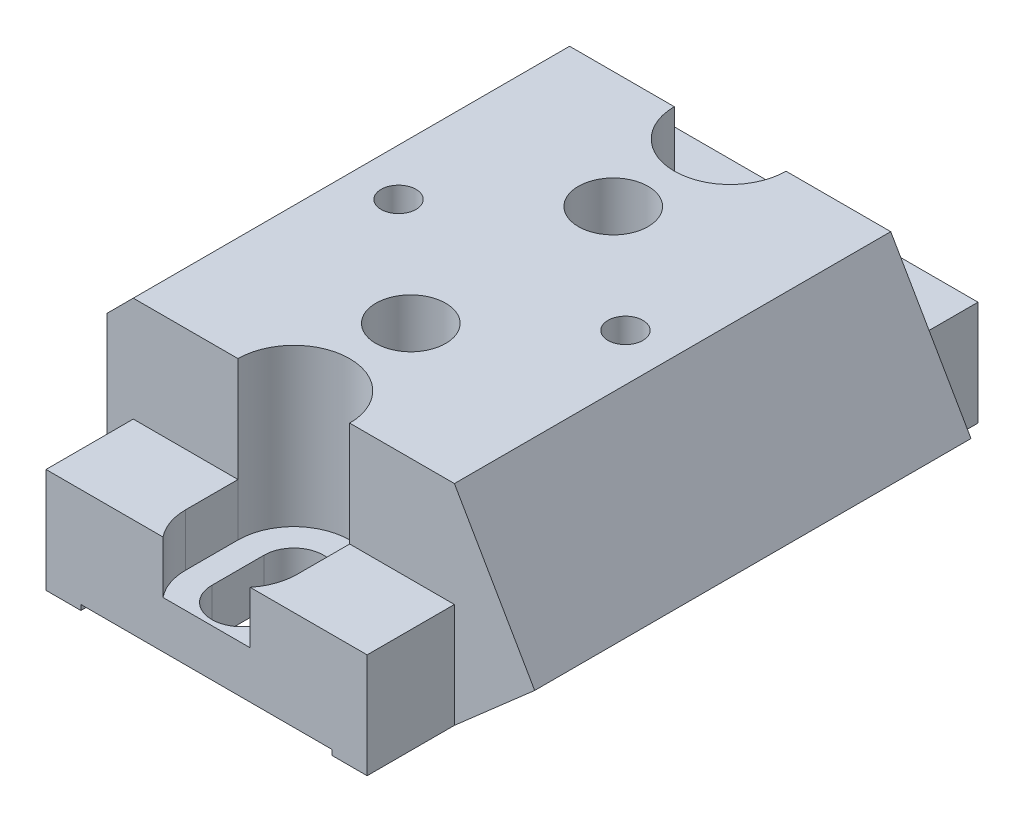
from build123d import *

# Parameters (mm, degrees)
SKETCH1_W           = 25
SKETCH1_H           = 12
BOSS_EXTRUDE1_DEPTH = 25
CUT_EXTRUDE1_DEPTH  = 30
CHAMFER1_SIZE       = 2
SKETCH5_W           = 21
SKETCH5_H           = 35
BOSS_EXTRUDE2_DEPTH = 6
SKETCH6_W           = 2.6
SKETCH6_H           = 5
CUT_EXTRUDE2_DEPTH  = 10
SKETCH11_W          = 14.4
SKETCH11_H          = 0.3
CUT_EXTRUDE5_DEPTH  = 48
CUT_EXTRUDE6_DEPTH  = 48
SKETCH15_W          = 25
SKETCH15_H          = 12
CUT_EXTRUDE8_DEPTH  = 0.5
SKETCH17_R          = 2
CUT_EXTRUDE10_DEPTH = 5
SKETCH18_R          = 1
CUT_EXTRUDE11_DEPTH = 4
CUT_EXTRUDE12_DEPTH = 17
CUT_EXTRUDE13_DEPTH = 9


with BuildPart() as part:
    # Sketch1 → Boss-Extrude1 (new body)
    with BuildSketch(Plane.XY):
        with Locations((12.5, -6)):
            Rectangle(SKETCH1_W, SKETCH1_H)
    extrude(amount=BOSS_EXTRUDE1_DEPTH)

    # Sketch2 → Cut-Extrude1 (cut)
    with BuildSketch(Plane.XY.offset(25)):
        Polygon((25, 0), (25, -7.967433715), (20.4, 0), align=None)
    extrude(amount=-CUT_EXTRUDE1_DEPTH, mode=Mode.SUBTRACT)

    # Chamfer1
    chamfer1_edges = [part.edges().sort_by_distance(p)[0] for p in [
        (0, 0, 12.5),
        (25, -12, 12.5),
        (0, -12, 12.5),
    ]]
    chamfer(chamfer1_edges, length=CHAMFER1_SIZE)

    # Sketch5 → Boss-Extrude2 (add)
    with BuildSketch(Plane.XZ.offset(12)):
        with Locations((12.5, 12.5)):
            Rectangle(SKETCH5_W, SKETCH5_H)
    extrude(amount=-BOSS_EXTRUDE2_DEPTH)

    # Sketch6 → Cut-Extrude2 (cut)
    with BuildSketch(Plane(origin=(0, -6, 0), x_dir=(1, 0, 0), z_dir=(0, 1, 0))):
        with Locations((21.7, -27.5)):
            Rectangle(SKETCH6_W, SKETCH6_H)
        with Locations((21.7, 2.5)):
            Rectangle(SKETCH6_W, SKETCH6_H)
    extrude(amount=-CUT_EXTRUDE2_DEPTH, mode=Mode.SUBTRACT)

    # Sketch11 → Cut-Extrude5 (cut)
    with BuildSketch(Plane.XY.offset(30)):
        with Locations((11.2, -11.85)):
            Rectangle(SKETCH11_W, SKETCH11_H)
    extrude(amount=-CUT_EXTRUDE5_DEPTH, mode=Mode.SUBTRACT)

    # Sketch12 → Cut-Extrude6 (cut)
    with BuildSketch(Plane.XY.offset(30)):
        Polygon((25, -7.967433715), (20.4, -12), (25.592855108, -12), align=None)
    extrude(amount=-CUT_EXTRUDE6_DEPTH, mode=Mode.SUBTRACT)

    # Sketch15 → Cut-Extrude8 (cut)
    with BuildSketch(Plane.ZY):
        with Locations((12.5, -6)):
            Rectangle(SKETCH15_W, SKETCH15_H)
    extrude(amount=-CUT_EXTRUDE8_DEPTH, mode=Mode.SUBTRACT)

    # Sketch17 → Cut-Extrude10 (cut)
    with BuildSketch(Plane(origin=(0, 0, 0), x_dir=(1, 0, 0), z_dir=(0, 1, 0))):
        with Locations(Location((11.2, -6.7, 0), (0, 0, 270))):
            Circle(SKETCH17_R)
        with Locations(Location((11.2, -18.3, 0), (0, 0, 270))):
            Circle(SKETCH17_R)
    extrude(amount=-CUT_EXTRUDE10_DEPTH, mode=Mode.SUBTRACT)

    # Sketch18 → Cut-Extrude11 (cut)
    with BuildSketch(Plane(origin=(0, 0, 0), x_dir=(1, 0, 0), z_dir=(0, 1, 0))):
        with Locations(Location((4.7, -12.5, 0), (0, 0, 270))):
            Circle(SKETCH18_R)
        with Locations(Location((17.7, -12.5, 0), (0, 0, 270))):
            Circle(SKETCH18_R)
    extrude(amount=-CUT_EXTRUDE11_DEPTH, mode=Mode.SUBTRACT)

    # Sketch19 → Cut-Extrude12 (cut)
    with BuildSketch(Plane(origin=(0, 0, 0), x_dir=(1, 0, 0), z_dir=(0, 1, 0))):
        with BuildLine():
            Line((12.9, -25), (12.9, -28))
            ThreePointArc((12.9, -28), (11.2, -29.7), (9.5, -28))
            Line((9.5, -28), (9.5, -25))
            ThreePointArc((9.5, -25), (11.2, -23.3), (12.9, -25))
        make_face()
        with BuildLine():
            Line((12.9, 0), (12.9, 3))
            ThreePointArc((12.9, 3), (11.2, 4.7), (9.5, 3))
            Line((9.5, 3), (9.5, 0))
            ThreePointArc((9.5, 0), (11.2, -1.7), (12.9, 0))
        make_face()
    extrude(amount=-CUT_EXTRUDE12_DEPTH, mode=Mode.SUBTRACT)

    # Sketch20 → Cut-Extrude13 (cut)
    with BuildSketch(Plane(origin=(0, 0, 0), x_dir=(1, 0, 0), z_dir=(0, 1, 0))):
        with BuildLine():
            Line((14.4, -25), (14.4, -28))
            ThreePointArc((14.4, -28), (11.2, -31.2), (8, -28))
            Line((8, -28), (8, -25))
            ThreePointArc((8, -25), (11.2, -21.8), (14.4, -25))
        make_face()
        with BuildLine():
            Line((14.4, 0), (14.4, 3))
            ThreePointArc((14.4, 3), (11.2, 6.2), (8, 3))
            Line((8, 3), (8, 0))
            ThreePointArc((8, 0), (11.2, -3.2), (14.4, 0))
        make_face()
    extrude(amount=-CUT_EXTRUDE13_DEPTH, mode=Mode.SUBTRACT)


solid = part.part
